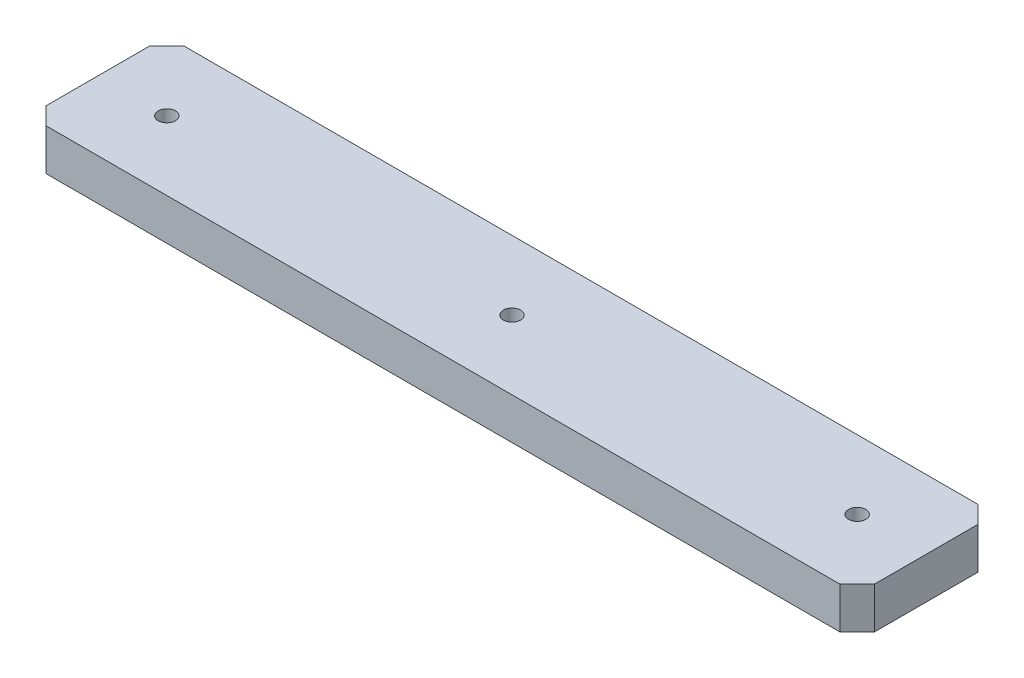
from build123d import *

# Parameters (mm, degrees)
SKETCH1_W             = 240
SKETCH1_H             = 40
EXTRUDE1_DEPTH        = 6
M6_TAPPED_HOLE1_D     = 5
M6_TAPPED_HOLE1_DEPTH = 15
M6_TAPPED_HOLE1_TIP   = 1.502151548
CHAMFER1_SIZE         = 5


with BuildPart() as part:
    # Sketch1 → Extrude1 (new, symmetric)
    with BuildSketch(Plane(origin=(0, 0, 0), x_dir=(1, 0, 0), z_dir=(0, 1, 0))):
        Rectangle(SKETCH1_W, SKETCH1_H)
    extrude(amount=EXTRUDE1_DEPTH, both=True)

    # M6 Tapped Hole1
    with Locations(Plane(origin=(0, 6, 0), x_dir=(-1, 0, 0), z_dir=(0, 1, 0))):
        with Locations((100, 0), (0, 0), (-100, 0)):
            Hole(M6_TAPPED_HOLE1_D / 2, depth=M6_TAPPED_HOLE1_DEPTH)
            with Locations((0, 0, -(M6_TAPPED_HOLE1_DEPTH + M6_TAPPED_HOLE1_TIP / 2))):  # 118° drill point
                Cone(0, M6_TAPPED_HOLE1_D / 2, M6_TAPPED_HOLE1_TIP, mode=Mode.SUBTRACT)

    # Chamfer1
    chamfer1_edges = [part.edges().sort_by_distance(p)[0] for p in [
        (-120, 0, -20),
        (120, 0, -20),
        (120, 0, 20),
        (-120, 0, 20),
    ]]
    chamfer(chamfer1_edges, length=CHAMFER1_SIZE)


solid = part.part
